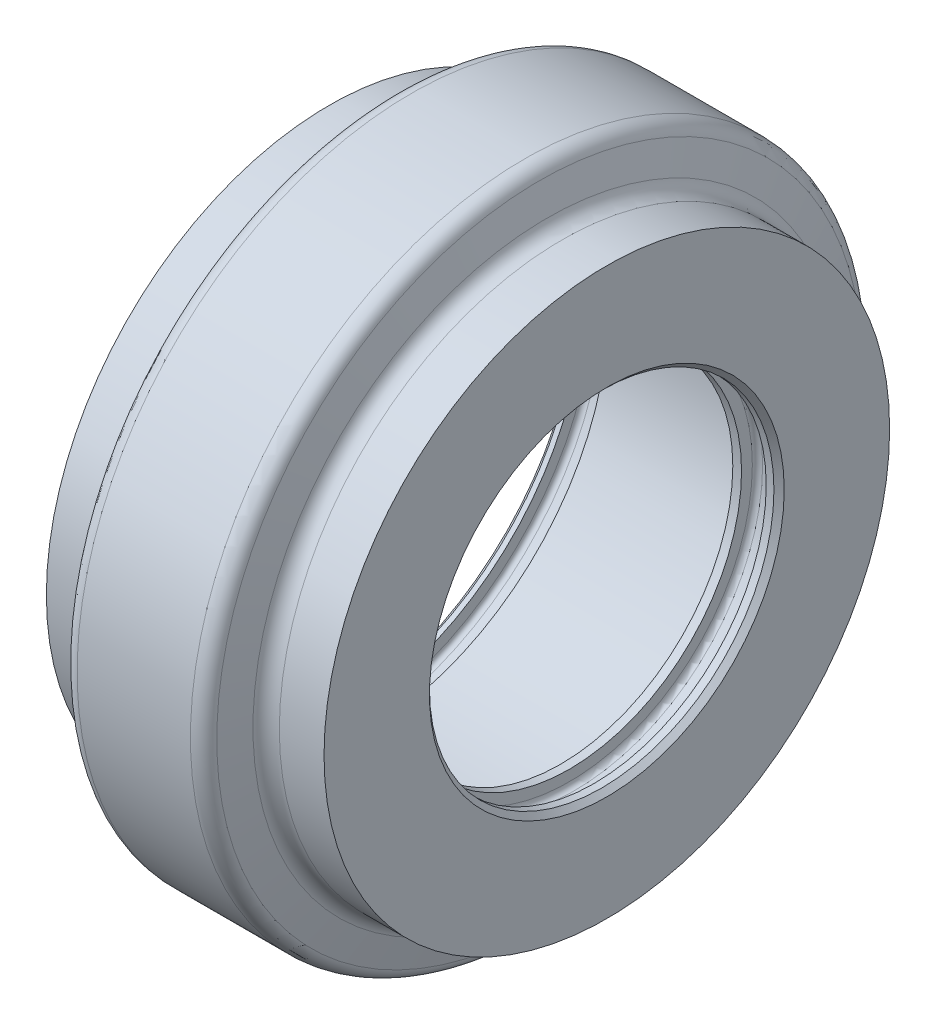
SolidWorks part; units mm, degrees
material "普通碳钢"
ref_plane "Front Plane" through (0, 0, 0) normal (0, 0, 1) x (1, 0, 0)
ref_plane "Top Plane" through (0, 0, 0) normal (0, 1, 0) x (1, 0, 0)
ref_plane "Right Plane" through (0, 0, 0) normal (1, 0, 0) x (0, 0, -1)
sketch "Sketch1" plane through (0, 0, 0) normal (0, 0, 1) x (1, 0, 0)
  line L0 (-27, 47.5) -> (-27, 55)
  line L1 (55, 0) -> (-55, 0) construction
  line L2 (-27, 55) -> (-18.302, 55)
  line L3 (-15.4042, 57.2235) -> (-13.9163, 62.7765)
  line L4 (-11.0185, 65) -> (11.0185, 65)
  line L5 (13.9163, 62.7765) -> (15.4042, 57.2235)
  line L6 (18.302, 55) -> (27, 55)
  line L7 (27, 55) -> (27, 33.5)
  line L8 (27, 0) -> (-27, 0) construction
  line L9 (0, 0) -> (0, 65) construction
  line L11 (-27, 47.5) -> (-25, 47.5)
  line L12 (-25, 47.5) -> (-25, 49.6)
  line L13 (-24, 50.6) -> (-21.2, 50.6)
  line L14 (-20.2, 49.6) -> (-20.2, 47.5)
  line L15 (-20.2, 47.5) -> (18, 47.5)
  line L20 (18, 47.5) -> (18, 33.5)
  line L21 (18, 33.5) -> (19.7, 33.5)
  line L22 (19.7, 33.5) -> (19.7, 35.6)
  line L23 (20.7, 36.6) -> (23.5, 36.6)
  line L24 (24.5, 35.6) -> (24.5, 33.5)
  line L25 (24.5, 33.5) -> (27, 33.5)
  line L26 (24.5, -33.5) -> (27, -33.5) construction
  line L27 (24.5, -36.6) -> (24.5, -33.5) construction
  line L28 (19.7, -36.6) -> (24.5, -36.6) construction
  line L29 (19.7, -33.5) -> (19.7, -36.6) construction
  line L30 (18, -33.5) -> (19.7, -33.5) construction
  line L36 (-20.2, -47.5) -> (18, -47.5) construction
  line L37 (-20.2, -50.6) -> (-20.2, -47.5) construction
  line L38 (-25, -50.6) -> (-20.2, -50.6) construction
  line L39 (-25, -47.5) -> (-25, -50.6) construction
  line L40 (-27, -47.5) -> (-25, -47.5) construction
  line L41 (27, -55) -> (27, -33.5) construction
  line L42 (16, -55) -> (27, -55) construction
  line L43 (13.3205, -65) -> (16, -55) construction
  line L44 (-13.3205, -65) -> (13.3205, -65) construction
  line L45 (-16, -55) -> (-13.3205, -65) construction
  line L46 (-27, -55) -> (-16, -55) construction
  line L47 (-27, -47.5) -> (-27, -55) construction
  arc A0 (-15.4042, 57.2235) -> (-18.302, 55) centre (-18.302, 58) cw
  arc A1 (-11.0185, 65) -> (-13.9163, 62.7765) centre (-11.0185, 62) ccw
  arc A2 (13.9163, 62.7765) -> (11.0185, 65) centre (11.0185, 62) ccw
  arc A3 (18.302, 55) -> (15.4042, 57.2235) centre (18.302, 58) cw
  arc A4 (24.5, 35.6) -> (23.5, 36.6) centre (23.5, 35.6) ccw
  arc A5 (20.7, 36.6) -> (19.7, 35.6) centre (20.7, 35.6) ccw
  arc A6 (-20.2, 49.6) -> (-21.2, 50.6) centre (-21.2, 49.6) ccw
  arc A7 (-24, 50.6) -> (-25, 49.6) centre (-24, 49.6) ccw
  point P24 (-20.2, 50.6)
  point P38 (-25, 50.6)
  point P55 (-16, 55)
  point P58 (-13.3205, 65)
  point P61 (13.3205, 65)
  point P64 (16, 55)
  point P65 (24.5, 36.6)
  point P68 (19.7, 36.6)
  dimension "D18" = 3
  dimension "D19" = 1
  dimension "D9" = 1
  dimension "D1" = 54
  dimension "D2" = 32
  dimension "D3" = 15
  dimension "D4" = 4.8
  dimension "D5" = 2.5
  dimension "D6" = 4.8
  dimension "D7" = 2
  dimension "D8" = 45
  dimension "D10" = 130
  dimension "D11" = 67
  dimension "D12" = 110
  dimension "D13" = 95
  dimension "D14" = 101.2
  dimension "D17" = 73.2
revolve "Revolve1" add sketch "Sketch1" angle 360 about L8
chamfer "Chamfer1" distance 1 angle 45 2 edges at (27, 0, -33.5) (-27, 0, -47.5)
